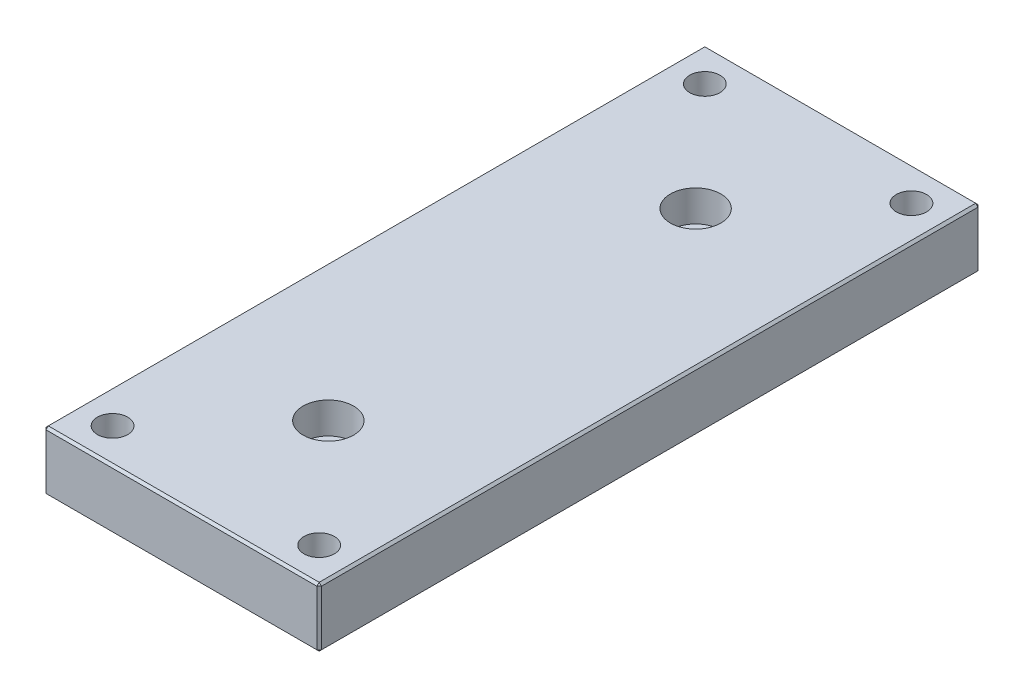
from build123d import *

# Parameters (mm, degrees)
SKETCH_1_W                  = 60
SKETCH_1_H                  = 13
EXTRUDE_1_DEPTH             = 144
HOLE_WIZARD_2_D             = 6.6
HOLE_WIZARD_2_CBORE_D       = 11
HOLE_WIZARD_2_CBORE_DEPTH   = 6.8
CHAMFER_1_SIZE              = 0.5
HOLE_WIZARD_2_2_D           = 6.6
HOLE_WIZARD_2_2_CBORE_D     = 11
HOLE_WIZARD_2_2_CBORE_DEPTH = 6.8


with BuildPart() as part:
    # 草图1 → 凸台-拉伸1 (new body)
    with BuildSketch(Plane.XY):
        Rectangle(SKETCH_1_W, SKETCH_1_H)
    extrude(amount=EXTRUDE_1_DEPTH)

    # Hole Wizard 2 (through all)
    with Locations(Plane(origin=(0, 6.5, 0), x_dir=(1, 0, 0), z_dir=(0, 1, 0))):
        with Locations((0, -32), (0, -112)):
            CounterBoreHole(HOLE_WIZARD_2_D / 2, HOLE_WIZARD_2_CBORE_D / 2, HOLE_WIZARD_2_CBORE_DEPTH)

    # 倒角1
    chamfer_1_edges = [part.edges().sort_by_distance(p)[0] for p in [
        (-30, 0, 144),
        (0, -6.5, 144),
        (30, 0, 144),
        (0, -6.5, 0),
        (-30, 0, 0),
        (0, 6.5, 0),
        (30, 0, 0),
        (0, 6.5, 144),
        (30, -6.5, 72),
        (-30, -6.5, 72),
        (-30, 6.5, 72),
        (30, 6.5, 72),
    ]]
    chamfer(chamfer_1_edges, length=CHAMFER_1_SIZE)

    # Hole Wizard 2 2 (through all)
    with Locations(Plane(origin=(0, -6.5, 0), x_dir=(-1, 0, 0), z_dir=(0, -1, 0))):
        with Locations((-22.5, -136.5), (22.5, -136.5), (-22.5, -7.5), (22.5, -7.5)):
            CounterBoreHole(HOLE_WIZARD_2_2_D / 2, HOLE_WIZARD_2_2_CBORE_D / 2, HOLE_WIZARD_2_2_CBORE_DEPTH)


solid = part.part
